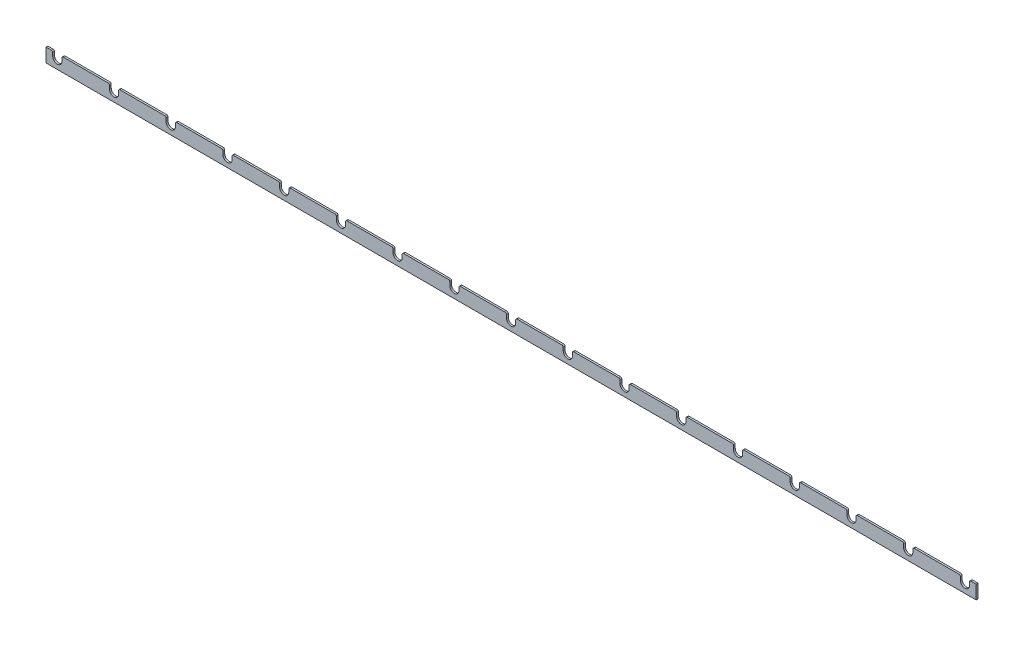
from build123d import *

# Parameters (mm, degrees)
SKETCH_1_W          = 2030
SKETCH_1_H          = 30
EXTRUDE_1_DEPTH     = 4
CUT_EXTRUDE_1_DEPTH = 4
FILLET_1_R          = 3


with BuildPart() as part:
    # 草图1 → 凸台-拉伸1 (new body)
    with BuildSketch(Plane.XY):
        Rectangle(SKETCH_1_W, SKETCH_1_H)
    extrude(amount=EXTRUDE_1_DEPTH)

    # 草图2 → 切除-拉伸1 (cut)
    with BuildSketch(Plane.XY.offset(4)):
        with BuildLine():
            Line((-1000.4, 5), (-1000.4, 15))
            Line((-1000.4, 15), (-980.4, 15))
            Line((-980.4, 15), (-980.4, 5))
            ThreePointArc((-980.4, 5), (-990.4, -5), (-1000.4, 5))
        make_face()
        with BuildLine():
            Line((-856.6, 15), (-876.6, 15))
            Line((-876.6, 15), (-876.6, 5))
            ThreePointArc((-876.6, 5), (-866.6, -5), (-856.6, 5))
            Line((-856.6, 5), (-856.6, 15))
        make_face()
        with BuildLine():
            Line((-732.8, 15), (-752.8, 15))
            Line((-752.8, 15), (-752.8, 5))
            ThreePointArc((-752.8, 5), (-742.8, -5), (-732.8, 5))
            Line((-732.8, 5), (-732.8, 15))
        make_face()
        with BuildLine():
            Line((-609, 15), (-629, 15))
            Line((-629, 15), (-629, 5))
            ThreePointArc((-629, 5), (-619, -5), (-609, 5))
            Line((-609, 5), (-609, 15))
        make_face()
        with BuildLine():
            Line((-485.2, 15), (-505.2, 15))
            Line((-505.2, 15), (-505.2, 5))
            ThreePointArc((-505.2, 5), (-495.2, -5), (-485.2, 5))
            Line((-485.2, 5), (-485.2, 15))
        make_face()
        with BuildLine():
            Line((-361.4, 15), (-381.4, 15))
            Line((-381.4, 15), (-381.4, 5))
            ThreePointArc((-381.4, 5), (-371.4, -5), (-361.4, 5))
            Line((-361.4, 5), (-361.4, 15))
        make_face()
        with BuildLine():
            Line((-237.6, 15), (-257.6, 15))
            Line((-257.6, 15), (-257.6, 5))
            ThreePointArc((-257.6, 5), (-247.6, -5), (-237.6, 5))
            Line((-237.6, 5), (-237.6, 15))
        make_face()
        with BuildLine():
            Line((-113.8, 15), (-133.8, 15))
            Line((-133.8, 15), (-133.8, 5))
            ThreePointArc((-133.8, 5), (-123.8, -5), (-113.8, 5))
            Line((-113.8, 5), (-113.8, 15))
        make_face()
        with BuildLine():
            Line((10, 15), (-10, 15))
            Line((-10, 15), (-10, 5))
            ThreePointArc((-10, 5), (0, -5), (10, 5))
            Line((10, 5), (10, 15))
        make_face()
        with BuildLine():
            Line((133.8, 15), (113.8, 15))
            Line((113.8, 15), (113.8, 5))
            ThreePointArc((113.8, 5), (123.8, -5), (133.8, 5))
            Line((133.8, 5), (133.8, 15))
        make_face()
        with BuildLine():
            Line((257.6, 15), (237.6, 15))
            Line((237.6, 15), (237.6, 5))
            ThreePointArc((237.6, 5), (247.6, -5), (257.6, 5))
            Line((257.6, 5), (257.6, 15))
        make_face()
        with BuildLine():
            Line((381.4, 15), (361.4, 15))
            Line((361.4, 15), (361.4, 5))
            ThreePointArc((361.4, 5), (371.4, -5), (381.4, 5))
            Line((381.4, 5), (381.4, 15))
        make_face()
        with BuildLine():
            Line((505.2, 15), (485.2, 15))
            Line((485.2, 15), (485.2, 5))
            ThreePointArc((485.2, 5), (495.2, -5), (505.2, 5))
            Line((505.2, 5), (505.2, 15))
        make_face()
        with BuildLine():
            Line((629, 15), (609, 15))
            Line((609, 15), (609, 5))
            ThreePointArc((609, 5), (619, -5), (629, 5))
            Line((629, 5), (629, 15))
        make_face()
        with BuildLine():
            Line((752.8, 15), (732.8, 15))
            Line((732.8, 15), (732.8, 5))
            ThreePointArc((732.8, 5), (742.8, -5), (752.8, 5))
            Line((752.8, 5), (752.8, 15))
        make_face()
        with BuildLine():
            Line((876.6, 15), (856.6, 15))
            Line((856.6, 15), (856.6, 5))
            ThreePointArc((856.6, 5), (866.6, -5), (876.6, 5))
            Line((876.6, 5), (876.6, 15))
        make_face()
        with BuildLine():
            Line((1000.4, 15), (980.4, 15))
            Line((980.4, 15), (980.4, 5))
            ThreePointArc((980.4, 5), (990.4, -5), (1000.4, 5))
            Line((1000.4, 5), (1000.4, 15))
        make_face()
    extrude(amount=-CUT_EXTRUDE_1_DEPTH, mode=Mode.SUBTRACT)

    # 圆角1
    fillet_1_edges = [part.edges().sort_by_distance(p)[0] for p in [
        (-876.6, 15, 2),
        (-856.6, 15, 2),
        (-752.8, 15, 2),
        (-732.8, 15, 2),
        (-629, 15, 2),
        (-609, 15, 2),
        (-505.2, 15, 2),
        (-485.2, 15, 2),
        (-381.4, 15, 2),
        (-361.4, 15, 2),
        (-257.6, 15, 2),
        (-237.6, 15, 2),
        (-133.8, 15, 2),
        (-113.8, 15, 2),
        (-10, 15, 2),
        (10, 15, 2),
        (113.8, 15, 2),
        (133.8, 15, 2),
        (237.6, 15, 2),
        (257.6, 15, 2),
        (361.4, 15, 2),
        (381.4, 15, 2),
        (485.2, 15, 2),
        (505.2, 15, 2),
        (609, 15, 2),
        (629, 15, 2),
        (732.8, 15, 2),
        (752.8, 15, 2),
        (856.6, 15, 2),
        (876.6, 15, 2),
        (980.4, 15, 2),
        (1000.4, 15, 2),
        (-1000.4, 15, 2),
        (-980.4, 15, 2),
    ]]
    fillet(fillet_1_edges, radius=FILLET_1_R)


solid = part.part
